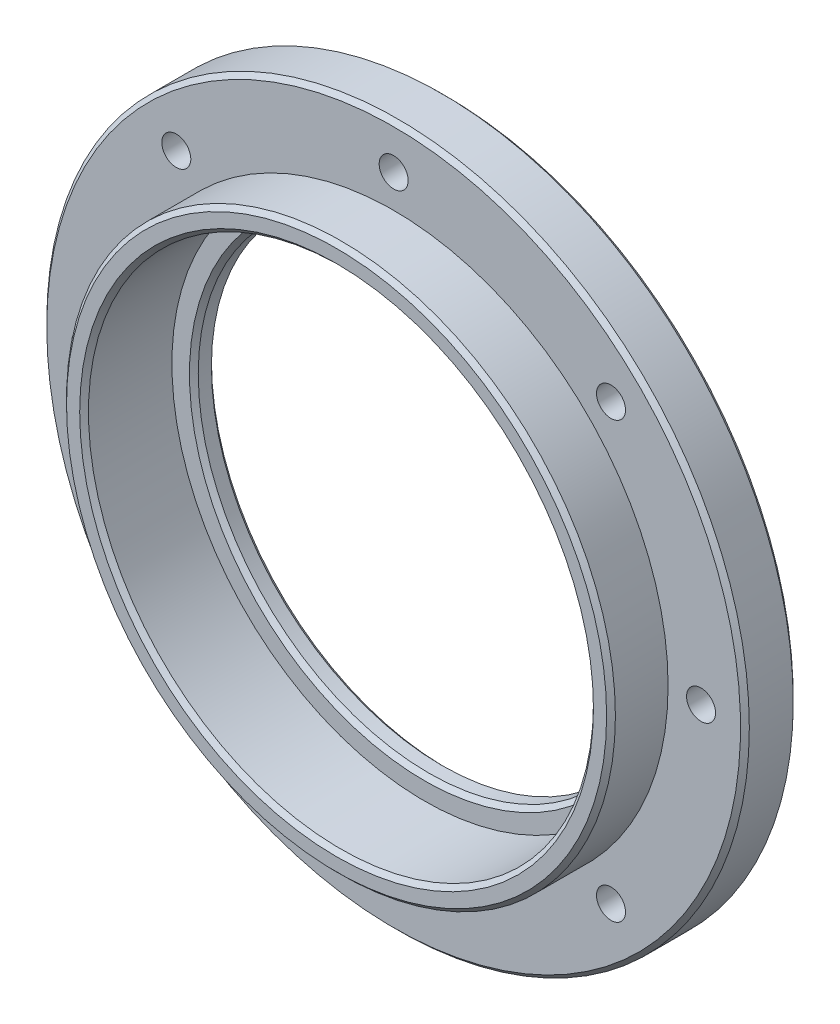
SolidWorks part; units mm, degrees
ref_plane "Front Plane" through (0, 0, 0) normal (0, 0, 1) x (1, 0, 0)
ref_plane "Top Plane" through (0, 0, 0) normal (0, 1, 0) x (1, 0, 0)
ref_plane "Right Plane" through (0, 0, 0) normal (1, 0, 0) x (0, 0, -1)
sketch "Sketch1" plane through (0, 0, 0) normal (0, 0, 1) x (1, 0, 0)
  circle A0 centre (0, 0) radius 57.5
  circle A1 centre (0, 0) radius 62.5
  dimension "D1" = 115
  dimension "D2" = 5
extrude "Boss-Extrude1" add sketch "Sketch1" along normal blind 13
sketch "Sketch2" plane through (0, 0, 0) normal (0, 0, -1) x (-1, 0, 0)
  circle A0 centre (0, 0) radius 80
  circle A1 centre (0, 0) radius 52.5
  dimension "D1" = 160
  dimension "D2" = 105
extrude "Boss-Extrude2" add sketch "Sketch2" along normal blind 12
sketch "Sketch3" plane through (0, 0, 0) normal (0, 0, 1) x (1, 0, 0)
  circle A0 centre (0, 0) radius 57.5
  dimension "D1" = 115
extrude "Cut-Extrude1" cut sketch "Sketch3" against normal blind 7
hole_wizard "Hole size (%based on) socket head cap screw type1" positions "Sketch4" profile "Sketch5" counterbore size "M6" standard "GB"
sketch "Sketch4" plane through (0, 0, -12) normal (0, 0, -1) x (-1, 0, 0)
  line L0 (0, 0) -> (70, 0) construction
  point P0 (70, 0)
  dimension "D1" = 70
sketch "Sketch5" plane through (-70, 0, -12) normal (1, 0, 0) x (0, 1, 0)
  line L0 (0, 0) -> (0, 26.4828)
  line L1 (0, 26.4828) -> (3.3, 24.5)
  line L2 (3.3, 24.5) -> (3.3, 6.8)
  line L3 (3.3, 6.8) -> (5.5, 6.8)
  line L4 (5.5, 6.8) -> (5.5, 0)
  line L5 (5.5, 0) -> (0, 0)
  line L10 (0, 26.4828) -> (-3.3, 24.5) construction
  line L11 (0, -6.35) -> (0, 107.95) construction
  dimension "孔直径" = 6.6
  dimension "孔深度" = 24.5
  dimension "柱形沉头孔直径" = 11
  dimension "柱形沉头孔深度" = 6.8
  dimension "导头角度" = 118
pattern_circular "CirPattern1" count 8 over 360 about axis through (0, 0, 0) along (0, 0, 1) of "Hole size (%based on) socket head cap screw type1"
chamfer "Chamfer1" distance 1 angle 45 6 edges at (52.5, 0, -7) (-52.5, 0, -12) (-80, 0, -12) (-80, 0, 0) (62.5, 0, 13) (57.5, 0, 13)
